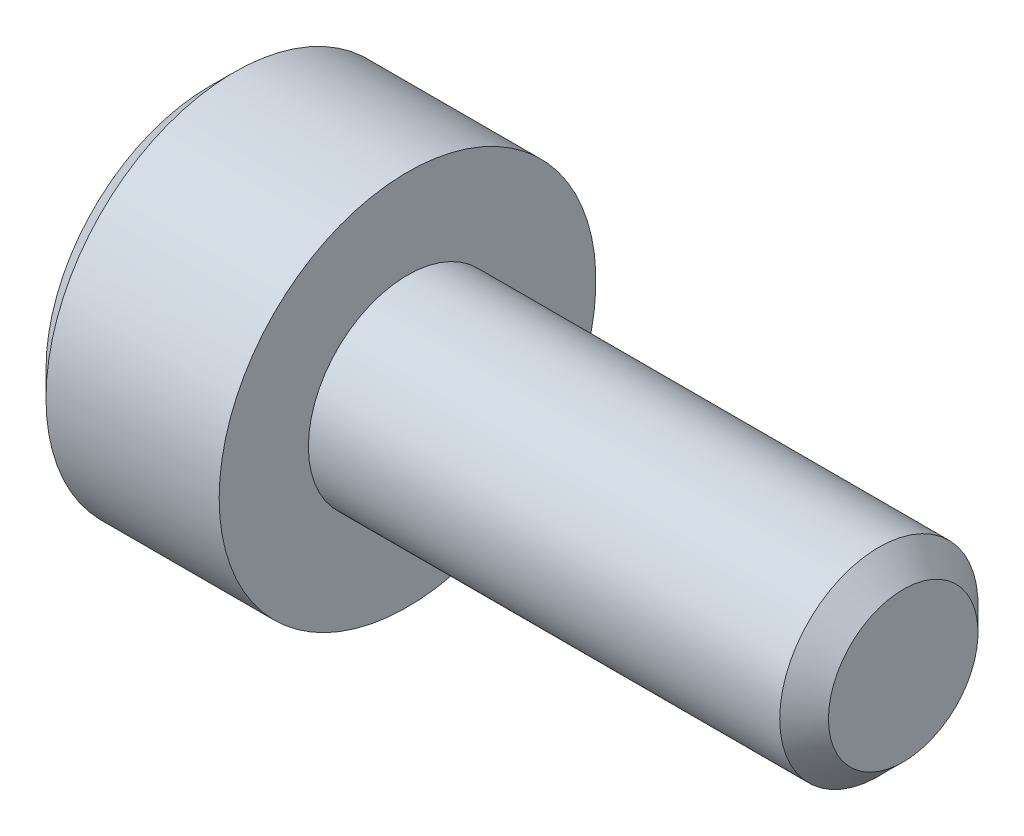
SolidWorks part; units mm, degrees
material "AISI 304"
ref_plane "Front Plane" through (0, 0, 0) normal (0, 0, 1) x (1, 0, 0)
ref_plane "Top Plane" through (0, 0, 0) normal (0, 1, 0) x (1, 0, 0)
ref_plane "Right Plane" through (0, 0, 0) normal (1, 0, 0) x (0, 0, -1)
sketch "Sketch1" plane through (0, 0, 0) normal (0, 0, 1) x (1, 0, 0)
  line L0 (-2, 0) -> (-2, 1.6467)
  line L1 (-2, 1.6467) -> (-1.7467, 1.9)
  line L2 (-1.7467, 1.9) -> (0, 1.9)
  line L3 (0, 1.9) -> (0, 1)
  line L4 (0, 1) -> (4.7543, 1)
  line L5 (4.7543, 1) -> (5, 0.7543)
  line L6 (5, 0.7543) -> (5, 0)
  line L7 (5, 0) -> (-2, 0)
  line L8 (5, 0) -> (-2, 0) construction
revolve "Revolve1" add sketch "Sketch1" angle 360 about L8
cosmetic thread "Cosmetic Thread1" parameters "D1"=4.5744, "D2"=1.5085
sketch "Sketch2" plane through (0, 0, 0) normal (0, 0, 1) x (1, 0, 0)
  line L0 (-2, 0) -> (-2, 0.75)
  line L1 (-2, 0.75) -> (-1, 0.75)
  line L2 (-1, 0.75) -> (-0.799, 0)
  line L3 (-0.799, 0) -> (-2, 0)
  line L4 (-0.799, 0) -> (-2, 0) construction
revolve "Cut-Revolve1" cut sketch "Sketch2" angle 360 about L4
ref_plane "Plane1" through (-2, 0, 0) normal (1, 0, 0) x (0, 0, -1)
sketch "Sketch3" plane through (-2, 0, 0) normal (1, 0, 0) x (0, 0, -1)
  line L0 (-0.75, 0.433) -> (-0.75, -0.433)
  line L1 (-0.75, -0.433) -> (0, -0.866)
  line L2 (0, -0.866) -> (0.75, -0.433)
  line L3 (0.75, -0.433) -> (0.75, 0.433)
  line L4 (0.75, 0.433) -> (0, 0.866)
  line L5 (0, 0.866) -> (-0.75, 0.433)
extrude "Cut-Extrude1" cut sketch "Sketch3" along normal blind 1
